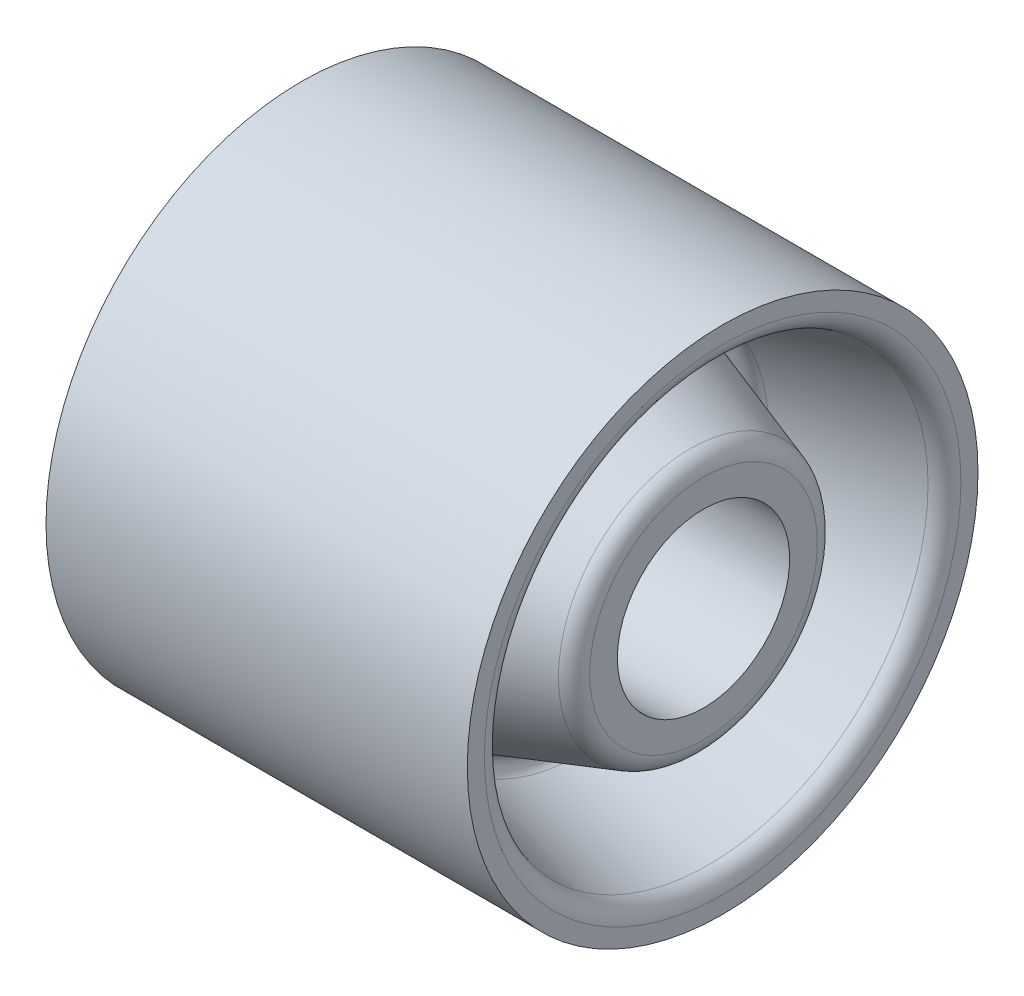
from build123d import *


with BuildPart() as part:
    # Sketch1 → Revolve1 (revolve)
    with BuildSketch(Plane.XY, mode=Mode.PRIVATE) as revolve1_sk:
        with BuildLine():
            Line((0, 40), (66, 40))
            Line((66, 40), (66, 37.321405707))
            ThreePointArc((66, 37.321405707), (65.372620854, 35.485467177), (63.752886476, 34.417415012))
            Line((63.752886476, 34.417415012), (43.906664603, 29.27209823))
            ThreePointArc((43.906664603, 29.27209823), (42.783976708, 27.871150368), (43.808766192, 26.397077936))
            Line((43.808766192, 26.397077936), (60.948683298, 20.683772234))
            ThreePointArc((60.948683298, 20.683772234), (62.433726556, 19.591853194), (63, 17.83772234))
            Line((63, 17.83772234), (63, 13.5))
            Line((63, 13.5), (3, 13.5))
            Line((3, 13.5), (3, 17.83772234))
            ThreePointArc((3, 17.83772234), (3.566273444, 19.591853194), (5.051316702, 20.683772234))
            Line((5.051316702, 20.683772234), (22.191233808, 26.397077936))
            ThreePointArc((22.191233808, 26.397077936), (23.216023292, 27.871150368), (22.093335397, 29.27209823))
            Line((22.093335397, 29.27209823), (2.247113524, 34.417415012))
            ThreePointArc((2.247113524, 34.417415012), (0.627379146, 35.485467177), (0, 37.321405707))
            Line((0, 37.321405707), (0, 40))
        make_face()
    revolve(revolve1_sk.sketch.rotate(Axis((0, 0, 0), (1, 0, 0)), 90), axis=Axis((0, 0, 0), (1, 0, 0)))


solid = part.part
